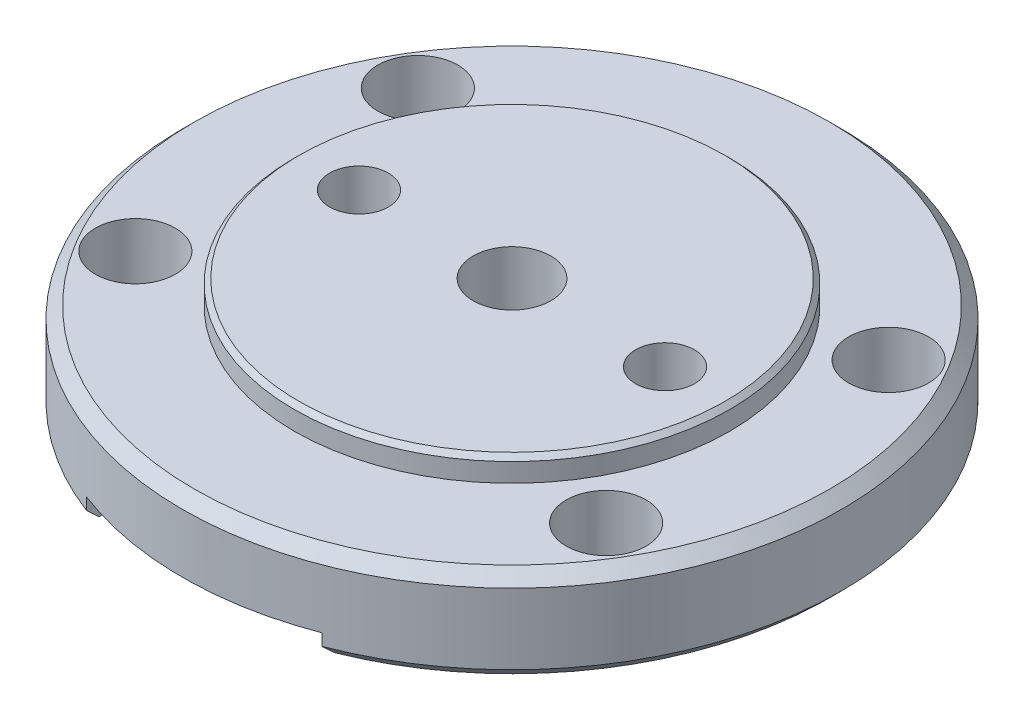
SolidWorks part; units mm, degrees
material "黑色铁氟龙 "
ref_plane "Front Plane" through (0, 0, 0) normal (0, 0, 1) x (1, 0, 0)
ref_plane "Top Plane" through (0, 0, 0) normal (0, 1, 0) x (1, 0, 0)
ref_plane "Right Plane" through (0, 0, 0) normal (1, 0, 0) x (0, 0, -1)
sketch "Sketch1" plane through (0, 0, 0) normal (0, 0, 1) x (1, 0, 0)
  line L0 (0, 0) -> (0, 15.9797) construction
  line L1 (0, 0) -> (14, 0)
  line L2 (14, 0) -> (14, 5)
  line L3 (14, 5) -> (6, 5)
  line L4 (6, 5) -> (6, 24)
  line L5 (6, 24) -> (4.5, 24)
  line L6 (4.5, 24) -> (4.5, 5)
  line L7 (4.5, 5) -> (0, 5)
  line L8 (0, 5) -> (0, 0)
  line L9 (4.5, 5) -> (6, 5)
  dimension "D1" = 14
  dimension "D2" = 5
  dimension "D3" = 24
  dimension "D4" = 4.5
  dimension "D5" = 1.5
revolve "Revolve1" add sketch "Sketch1" angle 360 about L0
hole_wizard "M3 Tapped Hole1" positions "Sketch12" profile "Sketch11" tap size "M3" standard "GB" end condition through all
sketch "Sketch12" plane through (0, 5, 0) normal (0, 1, 0) x (1, 0, 0)
  circle A0 centre (0, 0) radius 6.5 construction
  point P0 (-6.5, 0)
  point P2 (6.5, 0)
  dimension "D1" = 13
sketch "Sketch11" plane through (-6.5, 5, 0) normal (1, 0, 0) x (0, 0, 1)
  line L0 (0, 0) -> (0, 5)
  line L1 (0, 5) -> (1.25, 5)
  line L2 (1.25, 5) -> (1.25, 0)
  line L5 (1.25, 0) -> (0, 0)
  line L11 (0, -6.35) -> (0, 107.95) construction
  dimension "通孔螺纹孔钻头直径" = 2.5
  dimension "通孔螺纹孔钻头深度" = 5
cosmetic thread "Hole Thread2" parameters "D2"=3
cosmetic thread "Hole Thread3" parameters "D2"=3
sketch "Sketch3" plane through (0, 5, 0) normal (0, 1, 0) x (1, 0, 0)
  circle A0 centre (0, 0) radius 9.25
  dimension "D1" = 18.5
extrude "Cut-Extrude2" cut sketch "Sketch3" against normal blind 1 flip side to cut
hole_wizard "M3 Clearance Hole1" positions "Sketch5" profile "Sketch4" hole size "M3" standard "GB" end condition up to next
sketch "Sketch5" plane through (0, 0, 0) normal (0, -1, 0) x (-1, 0, 0)
  line L1 (-10, -6) -> (10, -6) construction
  line L2 (-10, -6) -> (-10, 6) construction
  line L3 (-10, 6) -> (10, 6) construction
  line L4 (10, -6) -> (10, 6) construction
  line L5 (-10, -6) -> (10, 6) construction
  line L6 (-10, 6) -> (10, -6) construction
  point P0 (10, -6)
  point P2 (10, 6)
  point P4 (-10, -6)
  point P6 (-10, 6)
  dimension "D1" = 20
  dimension "D2" = 12
sketch "Sketch4" plane through (-10, 0, 6) normal (1, 0, 0) x (0, 0, -1)
  line L0 (0, 0) -> (0, 4)
  line L1 (0, 4) -> (1.7, 4)
  line L2 (1.7, 4) -> (1.7, 0)
  line L5 (1.7, 0) -> (0, 0)
  line L11 (0, -6.35) -> (0, 107.95) construction
  dimension "通孔孔直径" = 3.4
  dimension "通孔孔深度" = 4
sketch "Sketch6" plane through (0, 0, 0) normal (0, -1, 0) x (1, 0, 0)
  line L1 (5, 15.7142) -> (-5, 15.7142)
  line L2 (5, 15.7142) -> (5, -15.7142)
  line L3 (5, -15.7142) -> (-5, -15.7142)
  line L4 (-5, 15.7142) -> (-5, -15.7142)
  line L5 (5, 15.7142) -> (-5, -15.7142) construction
  line L6 (5, -15.7142) -> (-5, 15.7142) construction
  point P0 (0, 0)
  dimension "D1" = 10
extrude "Cut-Extrude3" cut sketch "Sketch6" against normal blind 1
hole_wizard "M4 Tapped Hole1" positions "Sketch9" profile "Sketch8" tap size "M4" standard "GB" end condition up to next
sketch "Sketch9" plane through (0, 1, 0) normal (0, -1, 0) x (-1, 0, 0)
  point P0 (0, 0)
sketch "Sketch8" plane through (0, 1, 0) normal (1, 0, 0) x (0, 0, -1)
  line L0 (0, 0) -> (0, 4)
  line L1 (0, 4) -> (1.65, 4)
  line L2 (1.65, 4) -> (1.65, 0)
  line L5 (1.65, 0) -> (0, 0)
  line L11 (0, -6.35) -> (0, 107.95) construction
  dimension "通孔螺纹孔钻头直径" = 3.3
  dimension "通孔螺纹孔钻头深度" = 4
cosmetic thread "Hole Thread1" parameters "D2"=4
chamfer "Chamfer1" distance 0.5 angle 45 3 edges at (0, 4, 14) (14, 0, 0) (-14, 0, 0)
chamfer "Chamfer2" distance 0.2 angle 45 1 edges at (0, 5, 9.25)
